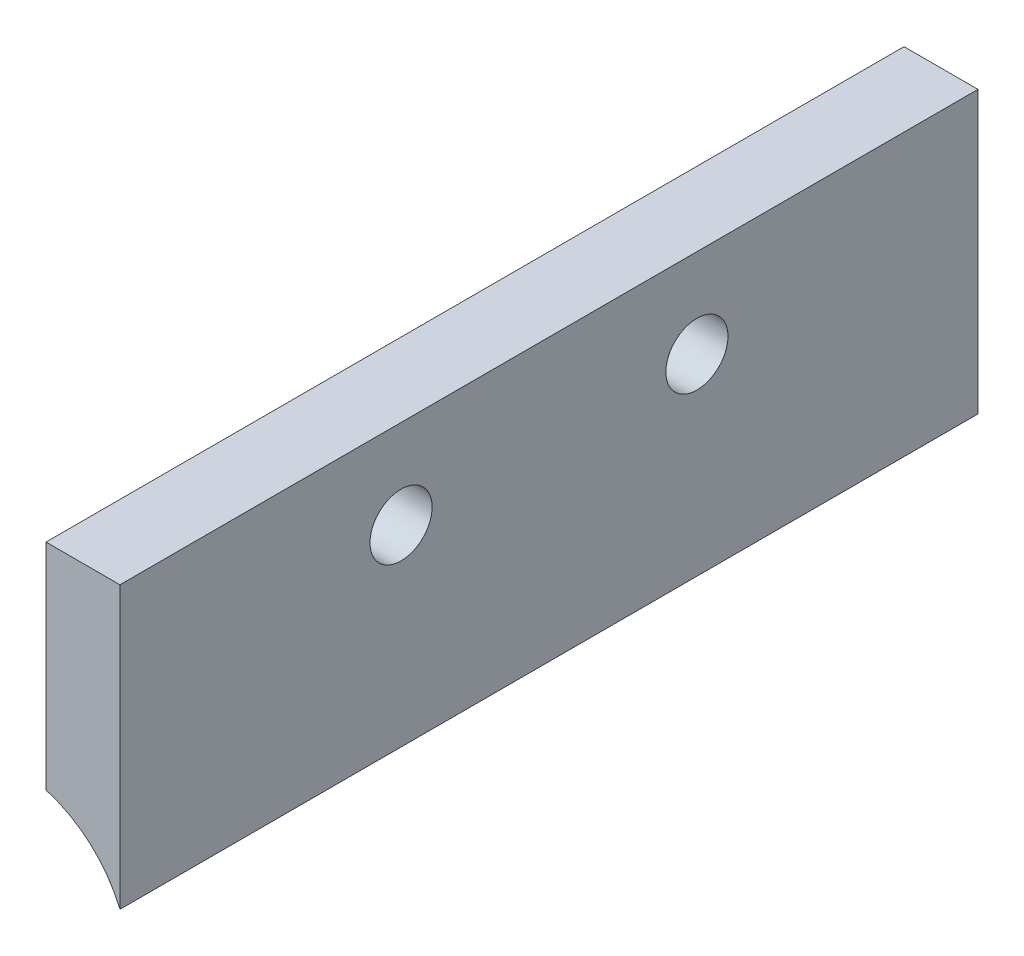
SolidWorks part; units mm, degrees
ref_plane "前视基准面" through (0, 0, 0) normal (0, 0, 1) x (1, 0, 0)
ref_plane "上视基准面" through (0, 0, 0) normal (0, 1, 0) x (1, 0, 0)
ref_plane "右视基准面" through (0, 0, 0) normal (1, 0, 0) x (0, 0, -1)
sketch "草图1" plane through (0, 0, 0) normal (0, 0, 1) x (1, 0, 0)
  line L1 (-2.7778, 6.0859) -> (2.2222, 6.0859)
  line L2 (-2.7778, 6.0859) -> (-2.7778, -8.4308)
  line L4 (2.2222, 6.0859) -> (2.2222, -12.9141)
  arc A0 (2.2222, -12.9141) -> (-2.7778, -8.4308) centre (-4.9778, -15.9141) ccw
  dimension "D3" = 15.6
  dimension "D1" = 5
  dimension "D2" = 19
extrude "凸台-拉伸1" add sketch "草图1" along normal blind 58
sketch "草图2" plane through (-2.7778, 0, 0) normal (-1, 0, 0) x (0, 0, 1)
  line L0 (0, 6.0859) -> (0, -8.4308) construction
  line L1 (58, 6.0859) -> (0, 6.0859) construction
  line L2 (58, 6.0859) -> (58, -8.4308) construction
  circle A0 centre (19, 0.0859) radius 2.1
  circle A1 centre (39, 0.0859) radius 2.1
  dimension "D1" = 4.2
  dimension "D2" = 4.2
  dimension "D3" = 19
  dimension "D4" = 6
  dimension "D5" = 19
  dimension "D6" = 6
extrude "切除-拉伸1" cut sketch "草图2" against normal through all
